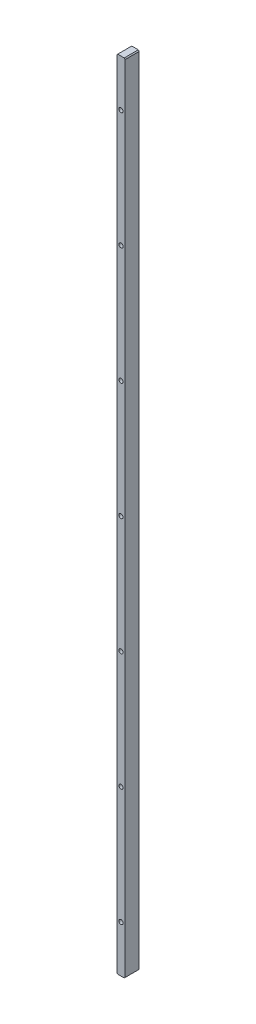
SolidWorks part; units mm, degrees
ref_plane "前视基准面" through (0, 0, 0) normal (0, 0, 1) x (1, 0, 0)
ref_plane "上视基准面" through (0, 0, 0) normal (0, 1, 0) x (1, 0, 0)
ref_plane "右视基准面" through (0, 0, 0) normal (1, 0, 0) x (0, 0, -1)
sketch "草图1" plane through (0, 0, 0) normal (0, 1, 0) x (1, 0, 0)
  line L1 (0, 0) -> (18, 0)
  line L2 (0, 0) -> (0, 30)
  line L3 (0, 30) -> (18, 30)
  line L4 (18, 0) -> (18, 30)
  dimension "D1" = 18
  dimension "D2" = 30
extrude "凸台-拉伸1" add sketch "草图1" along normal blind 1700
chamfer "倒角1" distance 2 angle 45 4 edges at (0, 0, -15) (0, 1700, -15) (18, 1700, -15) (18, 0, -15)
sketch "草图4" plane through (0, 0, -30) normal (0, 0, -1) x (-1, 0, 0)
  line L0 (-18, 850) -> (377.981, 850) construction
  line L1 (-18, 1698) -> (-18, 2) construction
  line L3 (-16, 1700) -> (-2, 1700) construction
  point P0 (-9, 1600)
  point P2 (-9, 1350)
  point P4 (-9, 1100)
  point P16 (-9, 1700)
  point P19 (-9, 600)
  point P20 (-9, 350)
  point P21 (-9, 100)
  point P22 (-9, 850)
  point P25 (0, 0)
  dimension "D1" = 250
  dimension "D2" = 500
  dimension "D3" = 250
hole_wizard "M8 六角圆柱头螺钉的柱形沉头孔1" positions "草图4" profile "草图3" counterbore size "M8" standard "GB" end condition through all
sketch "草图3" plane through (9, 1600, -30) normal (1, 0, 0) x (0, 1, 0)
  line L0 (0, 0) -> (0, 30)
  line L1 (0, 30) -> (4.5, 30)
  line L3 (4.5, 30) -> (4.5, 19)
  line L4 (4.5, 19) -> (7.5, 19)
  line L5 (7.5, 19) -> (7.5, 0)
  line L7 (7.5, 0) -> (0, 0)
  line L11 (0, -6.35) -> (0, 107.95) construction
  dimension "通孔孔直径" = 9
  dimension "通孔孔深度" = 30
  dimension "柱形沉头孔直径" = 15
  dimension "柱形沉头孔深度" = 19
